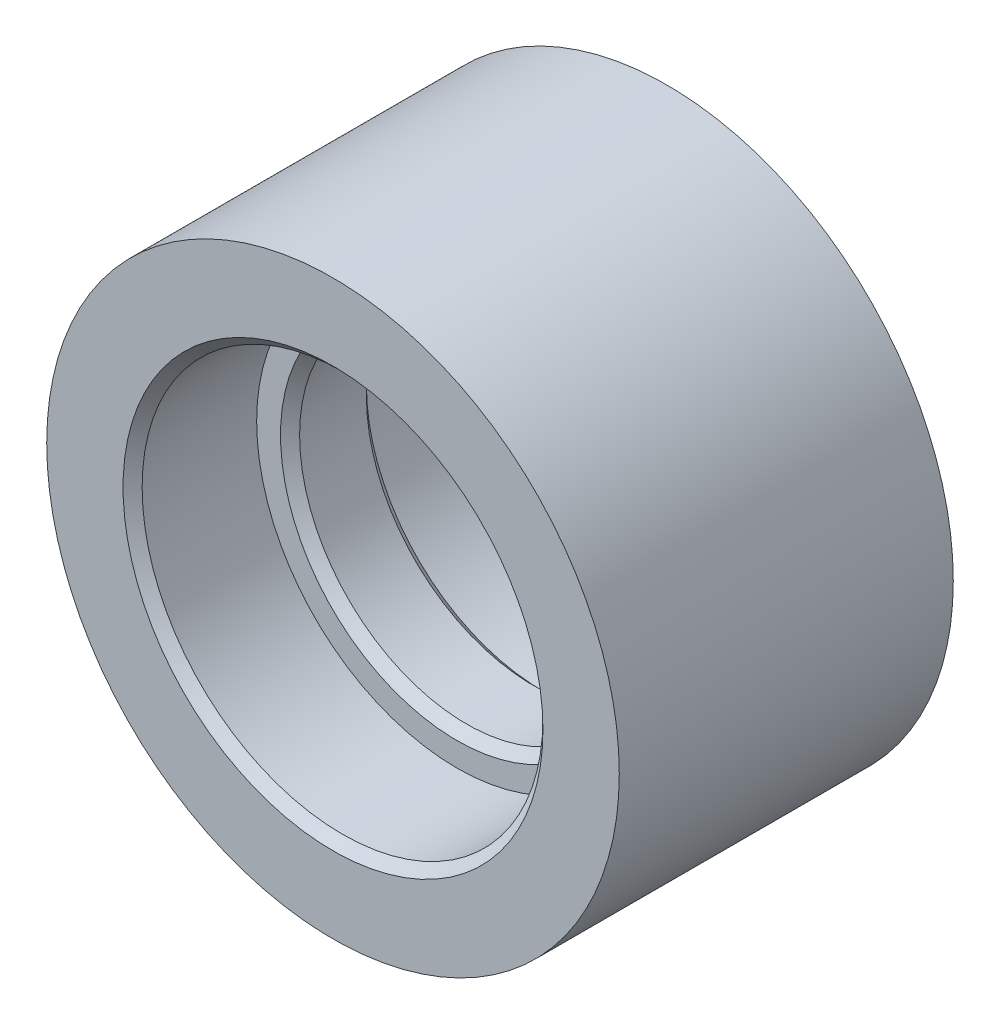
from build123d import *

# Parameters (mm, degrees)
SKETCH_1_R          = 30
SKETCH_1_R_2        = 17.5
EXTRUDE_1_DEPTH     = 17.5
SKETCH_2_R          = 21
CUT_EXTRUDE_1_DEPTH = 13
CHAMFER_1_SIZE      = 1


with BuildPart() as part:
    # 草图1 → 凸台-拉伸1 (new, symmetric)
    with BuildSketch(Plane.XY):
        Circle(SKETCH_1_R)
        Circle(SKETCH_1_R_2, mode=Mode.SUBTRACT)
    extrude(amount=EXTRUDE_1_DEPTH, both=True)

    # 草图2 → 切除-拉伸1 (cut)
    with BuildSketch(Plane.XY.offset(17.5)):
        Circle(SKETCH_2_R)
    cut_extrude_1 = extrude(amount=-CUT_EXTRUDE_1_DEPTH, mode=Mode.SUBTRACT)

    # 镜向1: 切除-拉伸1 across plane
    add(cut_extrude_1.mirror(Plane.XY), mode=Mode.SUBTRACT)

    # 倒角1
    chamfer_1_edges = [part.edges().sort_by_distance(p)[0] for p in [
        (-17.5, 0, 4.5),
        (-21, 0, 17.5),
        (-21, 0, -17.5),
        (-17.5, 0, -4.5),
    ]]
    chamfer(chamfer_1_edges, length=CHAMFER_1_SIZE)


solid = part.part
